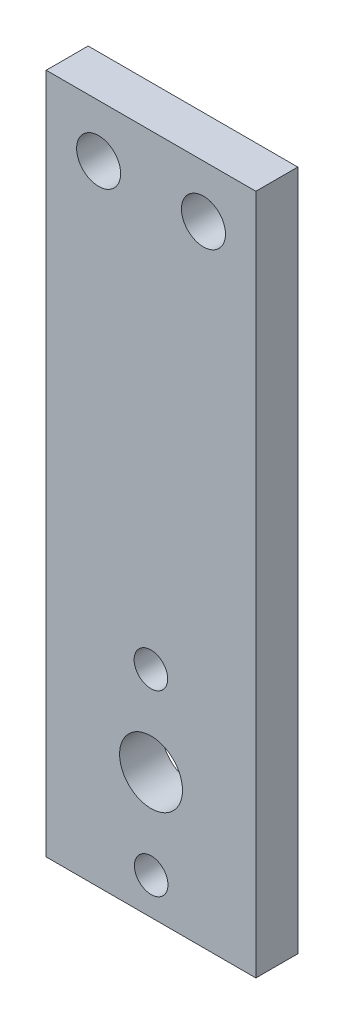
from build123d import *

# Parameters (mm, degrees)
SKETCH1_W           = 20
SKETCH1_H           = 65
SKETCH1_R           = 2.1
SKETCH1_R_2         = 3
SKETCH1_R_3         = 1.6
BOSS_EXTRUDE1_DEPTH = 4


with BuildPart() as part:
    # Sketch1 → Boss-Extrude1 (new body)
    with BuildSketch(Plane.XY):
        Rectangle(SKETCH1_W, SKETCH1_H)
        with Locations((-5, 27.5)):
            Circle(SKETCH1_R, mode=Mode.SUBTRACT)
        with Locations((5, 27.5)):
            Circle(SKETCH1_R, mode=Mode.SUBTRACT)
        with Locations((0, -20.5)):
            Circle(SKETCH1_R_2, mode=Mode.SUBTRACT)
        with Locations((-0.014007289, -12.000011541)):
            Circle(SKETCH1_R_3, mode=Mode.SUBTRACT)
        with Locations((0.014007289, -28.999988459)):
            Circle(SKETCH1_R_3, mode=Mode.SUBTRACT)
    extrude(amount=BOSS_EXTRUDE1_DEPTH)


solid = part.part
